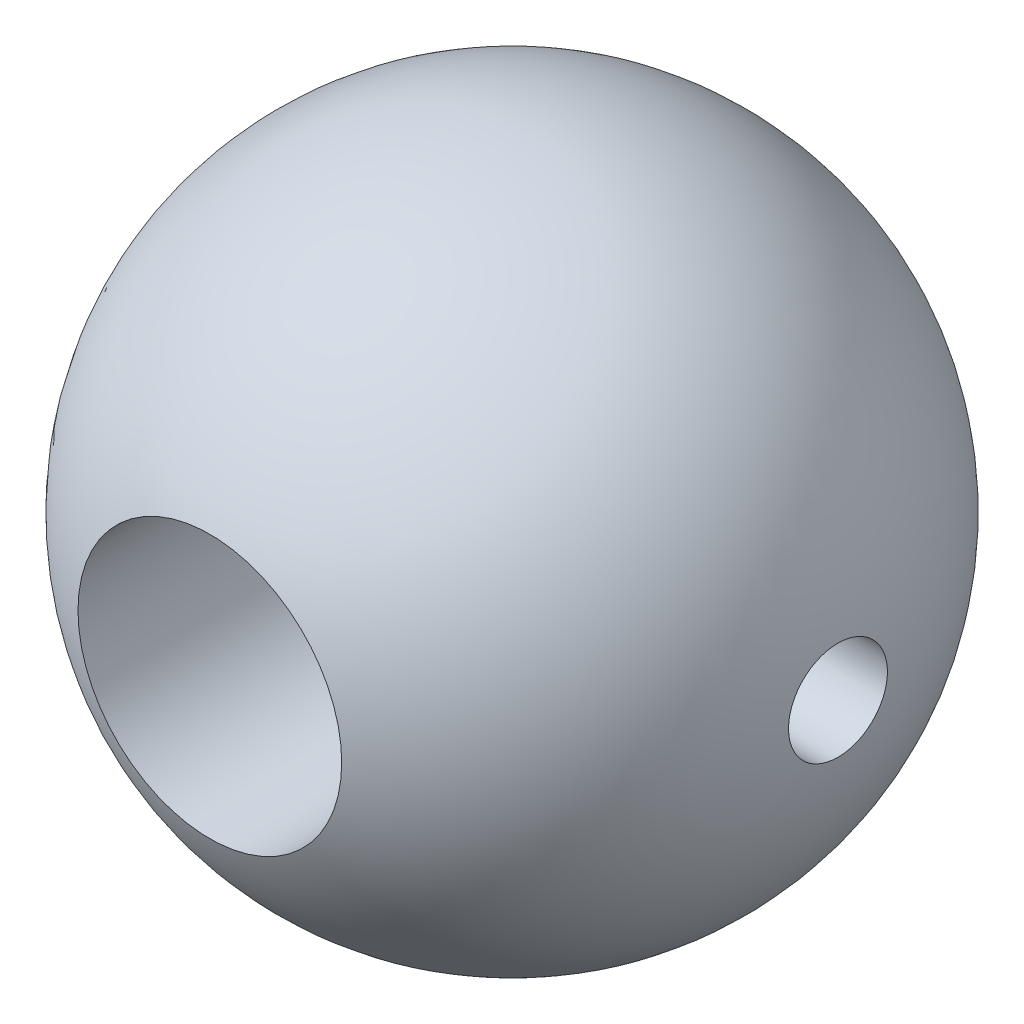
from build123d import *

# Parameters (mm, degrees)
SKETCH2_R          = 4
CUT_EXTRUDE1_DEPTH = 10
SKETCH3_R          = 1.5
CUT_EXTRUDE2_DEPTH = 15


with BuildPart() as part:
    # Sketch1 → Revolve1 (revolve)
    with BuildSketch(Plane.XY):
        with BuildLine():
            Line((0, 10), (0, -10))
            ThreePointArc((0, -10), (10, 0), (0, 10))
        make_face()
    revolve(axis=Axis((0, 10, 0), (0, -1, 0)))

    # Sketch2 → Cut-Extrude1 (cut, symmetric)
    with BuildSketch(Plane.XY):
        with Locations(Location((0, 0, 0), (0, 0, 180))):
            Circle(SKETCH2_R)
    extrude(amount=CUT_EXTRUDE1_DEPTH, both=True, mode=Mode.SUBTRACT)

    # Sketch3 → Cut-Extrude2 (cut, symmetric)
    with BuildSketch(Plane(origin=(0, 0, 0), x_dir=(0, 0, -1), z_dir=(1, 0, 0))):
        Circle(SKETCH3_R)
    extrude(amount=CUT_EXTRUDE2_DEPTH, both=True, mode=Mode.SUBTRACT)


solid = part.part
